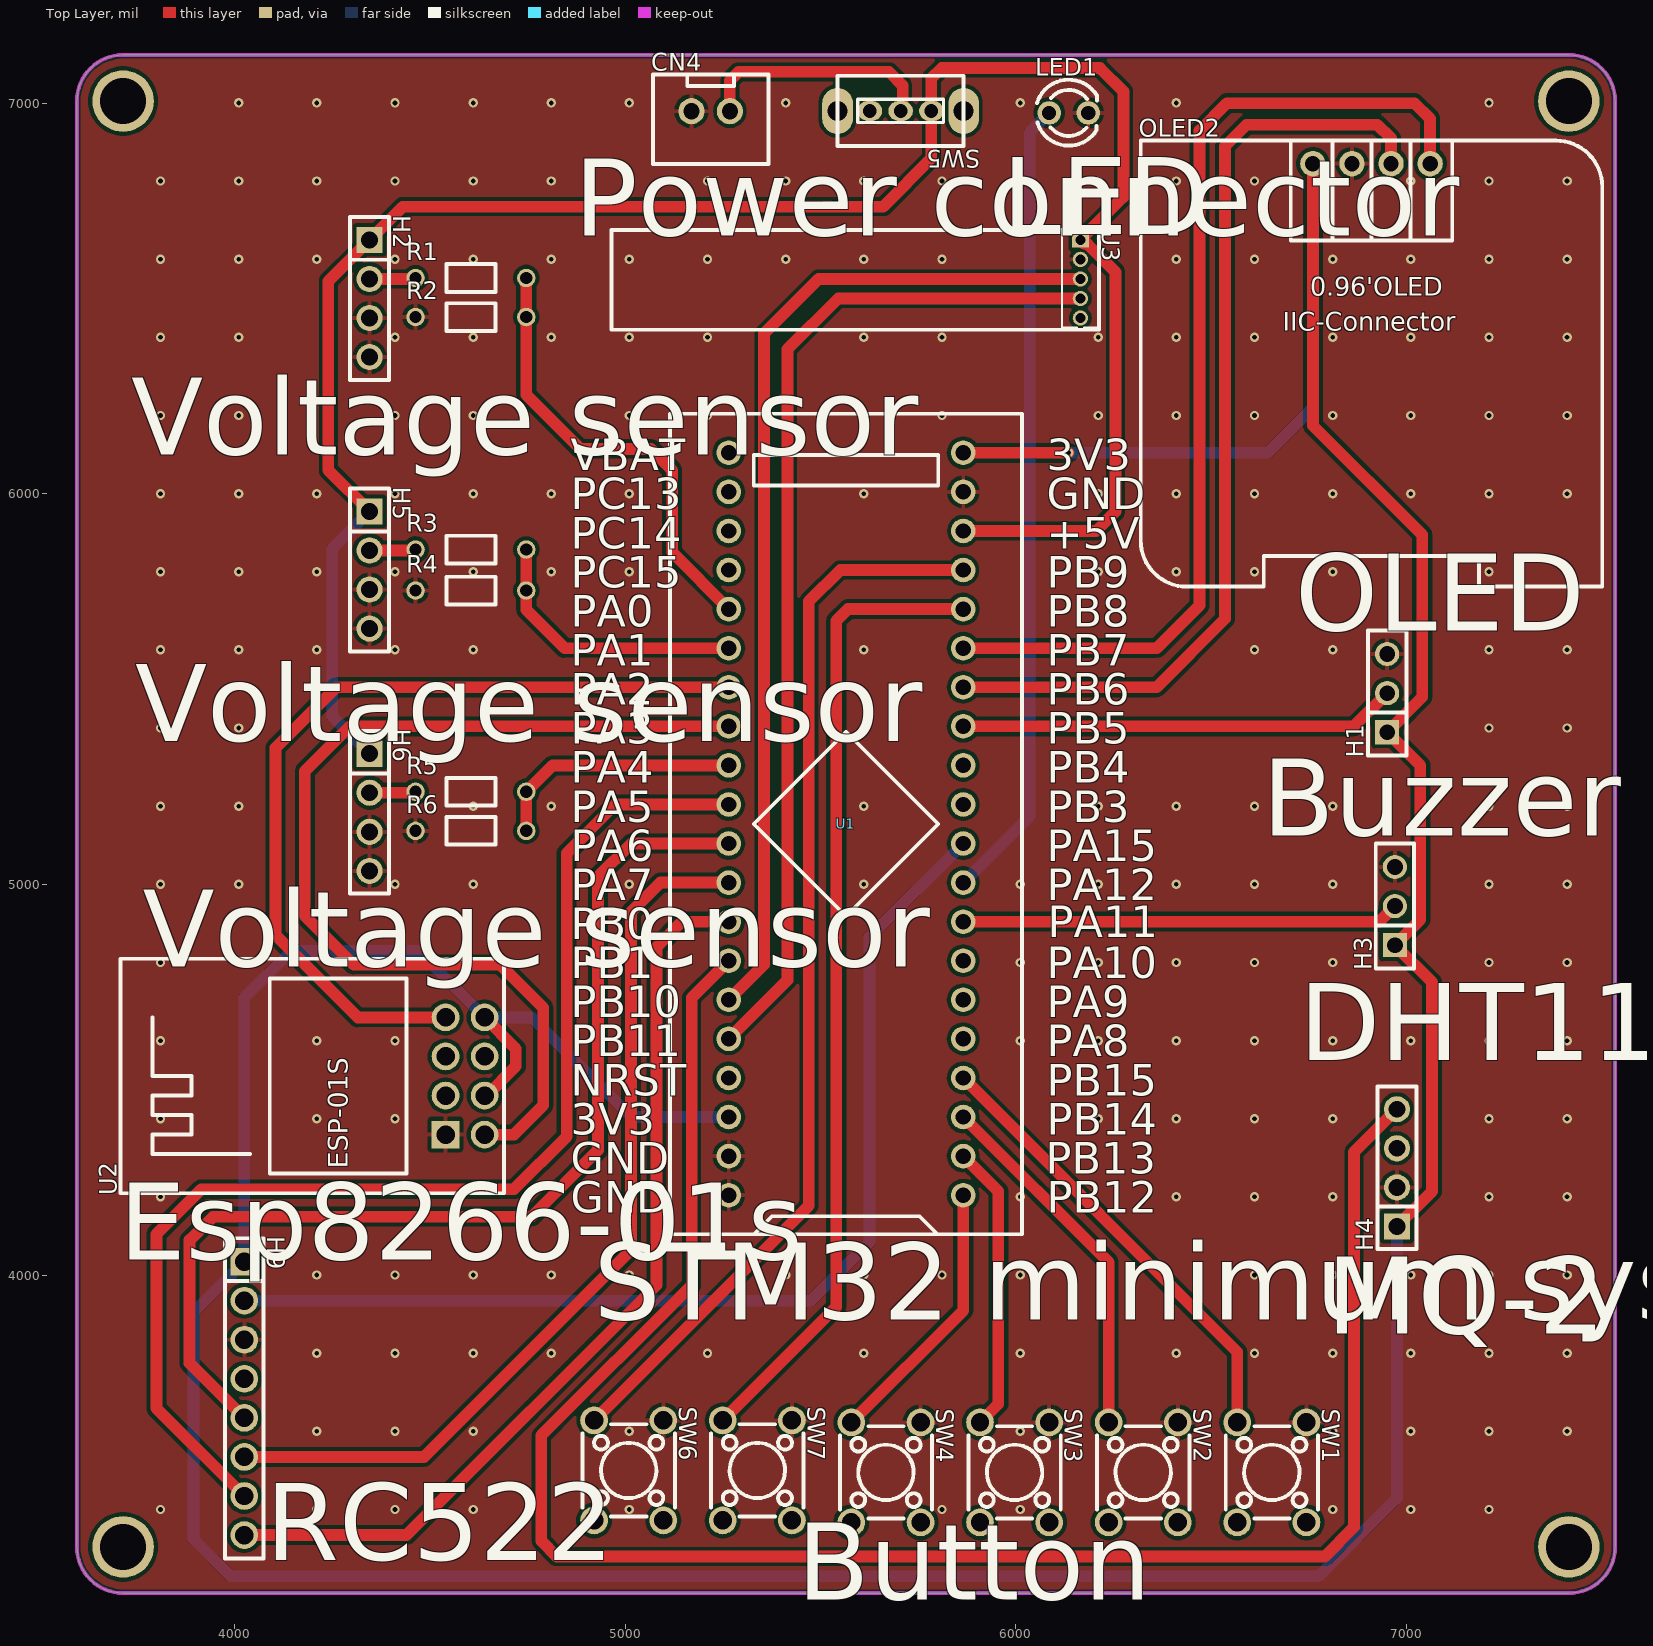
[diagram p0: Top Layer view]
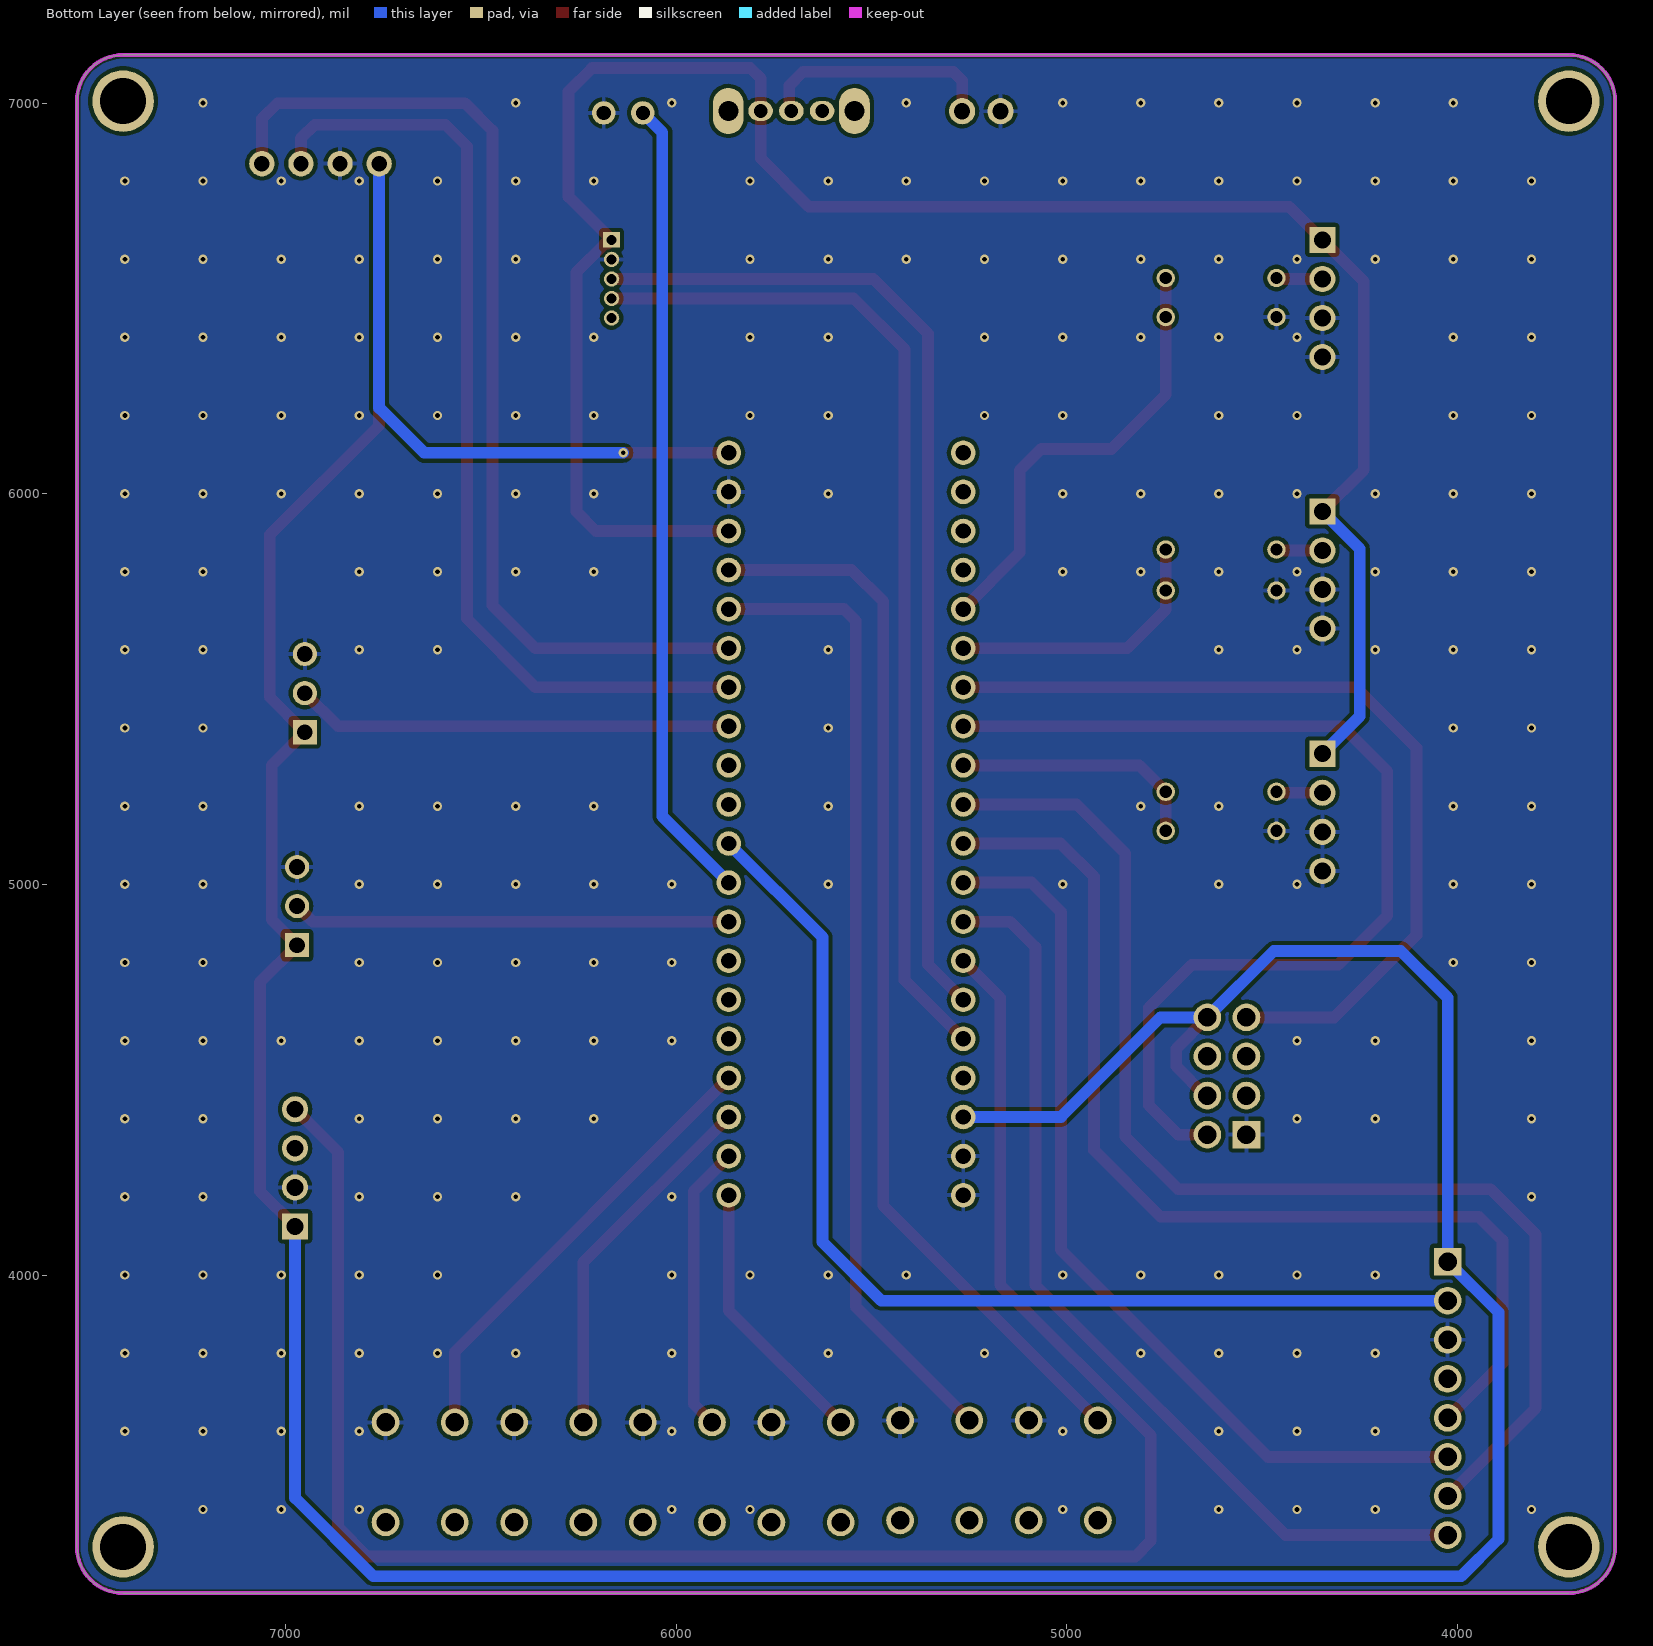
[diagram p1: Bottom Layer view, seen from below]
# Altium PCB MISC89009.pcbdoc
Units mil, origin at the board's own origin, x right, y up, seen from the top; angles counter-clockwise.
Board outline 3937.01 x 3937.01 mil, 2 copper layers (Top Layer, Bottom Layer), stack 62.206 mil thick; 26 components, 41 nets, 136 pads, 226 vias.

## Layer stack, top to bottom
Top Solder Mask Layer: solder mask 0.394, Dk 3.3
Top Layer: signal copper 1.379
Dielectric1: surface 59.449, FR4, Dk 4.5
Bottom Layer: signal copper 1.378
Bottom Solder Mask Layer: solder mask 0.394, Dk 3.3

## Board outline
3714.61,7123.5 ccw(c3714.61,7005.39) 3596.5,7005.39 3596.5,3304.61 ccw(c3714.61,3304.61) 3714.61,3186.5 7415.39,3186.5 ccw(c7415.39,3304.61) 7533.5,3304.61 7533.5,7005.39 ccw(c7415.39,7005.39) 7415.39,7123.5 3714.61,7123.5

## Design rules (kind name [scope] priority, off if disabled: settings)
BoardOutlineClearance copperThickness2oz_1 [All] p2 off: genericclearance=7.99 ignorepadtopadclearanceinfootprint=FALSE except(0: Arc-SplitContinuation Track-SplitContinuation SMDPad-SplitContinuation THPad-SplitContinuation Via-SplitContinuation Fill-SplitContinuation Region-SplitContinuation Poly-SplitContinuation Text-SplitContinuation Hole-SplitContinuation; 5.98: Arc-CutoutEdge Track-CutoutEdge SMDPad-CutoutEdge THPad-CutoutEdge Via-CutoutEdge Text-CutoutEdge; 6.9: Hole-OutlineEdge Hole-CutoutEdge; 10: Poly-OutlineEdge Poly-CutoutEdge; 11.81: Arc-OutlineEdge Track-OutlineEdge SMDPad-OutlineEdge THPad-OutlineEdge Via-OutlineEdge Fill-OutlineEdge Region-OutlineEdge Text-OutlineEdge Fill-CutoutEdge Region-CutoutEdge)
BoardOutlineClearance Plane_innerPlane_1 [All] p4 off: genericclearance=4.02 ignorepadtopadclearanceinfootprint=FALSE except(0: Arc-SplitContinuation Track-SplitContinuation SMDPad-SplitContinuation THPad-SplitContinuation Via-SplitContinuation Fill-SplitContinuation Region-SplitContinuation Poly-SplitContinuation Text-SplitContinuation Hole-SplitContinuation; 5.98: Arc-CutoutEdge Track-CutoutEdge SMDPad-CutoutEdge THPad-CutoutEdge Via-CutoutEdge Text-CutoutEdge; 6.9: Hole-OutlineEdge Hole-CutoutEdge; 10: Poly-OutlineEdge Poly-CutoutEdge; 11.81: Arc-OutlineEdge Track-OutlineEdge SMDPad-OutlineEdge THPad-OutlineEdge Via-OutlineEdge Fill-OutlineEdge Region-OutlineEdge Text-OutlineEdge Fill-CutoutEdge Region-CutoutEdge)
BoardOutlineClearance Copper_copperRegion_1 [All] p6 off: genericclearance=4.02 ignorepadtopadclearanceinfootprint=FALSE except(0: Arc-SplitContinuation Track-SplitContinuation SMDPad-SplitContinuation THPad-SplitContinuation Via-SplitContinuation Fill-SplitContinuation Region-SplitContinuation Poly-SplitContinuation Text-SplitContinuation Hole-SplitContinuation; 5.98: Arc-CutoutEdge Track-CutoutEdge SMDPad-CutoutEdge THPad-CutoutEdge Via-CutoutEdge Text-CutoutEdge; 6.9: Hole-OutlineEdge Hole-CutoutEdge; 10: Poly-OutlineEdge Poly-CutoutEdge; 11.81: Arc-OutlineEdge Track-OutlineEdge SMDPad-OutlineEdge THPad-OutlineEdge Via-OutlineEdge Fill-OutlineEdge Region-OutlineEdge Text-OutlineEdge Fill-CutoutEdge Region-CutoutEdge)
BoardOutlineClearance Copper_copperRegion_copperThickness1oz_1 [All] p8 off: genericclearance=4.02 ignorepadtopadclearanceinfootprint=FALSE except(0: Arc-SplitContinuation Track-SplitContinuation SMDPad-SplitContinuation THPad-SplitContinuation Via-SplitContinuation Fill-SplitContinuation Region-SplitContinuation Poly-SplitContinuation Text-SplitContinuation Hole-SplitContinuation; 5.98: Arc-CutoutEdge Track-CutoutEdge SMDPad-CutoutEdge THPad-CutoutEdge Via-CutoutEdge Text-CutoutEdge; 6.9: Hole-OutlineEdge Hole-CutoutEdge; 10: Poly-OutlineEdge Poly-CutoutEdge; 11.81: Arc-OutlineEdge Track-OutlineEdge SMDPad-OutlineEdge THPad-OutlineEdge Via-OutlineEdge Fill-OutlineEdge Region-OutlineEdge Text-OutlineEdge Fill-CutoutEdge Region-CutoutEdge)
BoardOutlineClearance Copper_copperRegion_Copper_copperRegion_1 [All] p10 off: genericclearance=4.02 ignorepadtopadclearanceinfootprint=FALSE except(0: Arc-SplitContinuation Track-SplitContinuation SMDPad-SplitContinuation THPad-SplitContinuation Via-SplitContinuation Fill-SplitContinuation Region-SplitContinuation Poly-SplitContinuation Text-SplitContinuation Hole-SplitContinuation; 5.98: Arc-CutoutEdge Track-CutoutEdge SMDPad-CutoutEdge THPad-CutoutEdge Via-CutoutEdge Text-CutoutEdge; 6.9: Hole-OutlineEdge Hole-CutoutEdge; 10: Poly-OutlineEdge Poly-CutoutEdge; 11.81: Arc-OutlineEdge Track-OutlineEdge SMDPad-OutlineEdge THPad-OutlineEdge Via-OutlineEdge Fill-OutlineEdge Region-OutlineEdge Text-OutlineEdge Fill-CutoutEdge Region-CutoutEdge)
BoardOutlineClearance copperThickness1oz_1 [All] p12: genericclearance=4.02 ignorepadtopadclearanceinfootprint=FALSE except(0: Arc-SplitContinuation Track-SplitContinuation SMDPad-SplitContinuation THPad-SplitContinuation Via-SplitContinuation Fill-SplitContinuation Region-SplitContinuation Poly-SplitContinuation Text-SplitContinuation Hole-SplitContinuation; 5.98: Arc-CutoutEdge Track-CutoutEdge SMDPad-CutoutEdge THPad-CutoutEdge Via-CutoutEdge Text-CutoutEdge; 6.9: Hole-OutlineEdge Hole-CutoutEdge; 10: Poly-OutlineEdge Poly-CutoutEdge; 11.81: Arc-OutlineEdge Track-OutlineEdge SMDPad-OutlineEdge THPad-OutlineEdge Via-OutlineEdge Fill-OutlineEdge Region-OutlineEdge Text-OutlineEdge Fill-CutoutEdge Region-CutoutEdge)
Clearance copperThickness2oz [All] p1 off: gap=7.99 ignorepadtopadclearanceinfootprint=FALSE except(5.98: SMDPad-Track SMDPad-SMDPad THPad-Track SMDPad-THPad THPad-THPad Track-Via SMDPad-Via THPad-Via Via-Via Fill-SMDPad Region-SMDPad Fill-THPad Region-THPad Fill-Via Region-Via Fill-Fill Fill-Region Region-Region Arc-Track Arc-SMDPad Arc-THPad Arc-Via Fill-Arc Region-Arc Arc-Arc Text-Track SMDPad-Text Text-THPad Text-Via Fill-Text Region-Text Arc-Text Text-Text; 6.9: Hole-Track Hole-SMDPad Hole-THPad Hole-Via Fill-Hole Region-Hole Hole-Arc Hole-Text; 10: Poly-Track Poly-SMDPad Poly-THPad Poly-Via Poly-Fill Poly-Region Poly-Poly Poly-Arc Poly-Text Poly-Hole; 11.81: Fill-Track Region-Track)
Clearance Plane_innerPlane [All] p3 off: gap=4.02 ignorepadtopadclearanceinfootprint=FALSE except(5.98: SMDPad-Track SMDPad-SMDPad THPad-Track SMDPad-THPad THPad-THPad Track-Via SMDPad-Via THPad-Via Via-Via Fill-SMDPad Region-SMDPad Fill-THPad Region-THPad Fill-Via Region-Via Fill-Fill Fill-Region Region-Region Arc-Track Arc-SMDPad Arc-THPad Arc-Via Fill-Arc Region-Arc Arc-Arc Text-Track SMDPad-Text Text-THPad Text-Via Fill-Text Region-Text Arc-Text Text-Text; 6.9: Hole-Track Hole-SMDPad Hole-THPad Hole-Via Fill-Hole Region-Hole Hole-Arc Hole-Text; 10: Poly-Track Poly-SMDPad Poly-THPad Poly-Via Poly-Fill Poly-Region Poly-Poly Poly-Arc Poly-Text Poly-Hole; 11.81: Fill-Track Region-Track)
Clearance Copper_copperRegion [All] p5 off: gap=4.02 ignorepadtopadclearanceinfootprint=FALSE except(5.98: SMDPad-Track SMDPad-SMDPad THPad-Track SMDPad-THPad THPad-THPad Track-Via SMDPad-Via THPad-Via Via-Via Fill-SMDPad Region-SMDPad Fill-THPad Region-THPad Fill-Via Region-Via Fill-Fill Fill-Region Region-Region Arc-Track Arc-SMDPad Arc-THPad Arc-Via Fill-Arc Region-Arc Arc-Arc Text-Track SMDPad-Text Text-THPad Text-Via Fill-Text Region-Text Arc-Text Text-Text; 6.9: Hole-Track Hole-SMDPad Hole-THPad Hole-Via Fill-Hole Region-Hole Hole-Arc Hole-Text; 10: Poly-Track Poly-SMDPad Poly-THPad Poly-Via Poly-Fill Poly-Region Poly-Poly Poly-Arc Poly-Text Poly-Hole; 11.81: Fill-Track Region-Track)
Clearance Copper_copperRegion_copperThickness1oz [All] p7 off: gap=4.02 ignorepadtopadclearanceinfootprint=FALSE except(5.98: SMDPad-Track SMDPad-SMDPad THPad-Track SMDPad-THPad THPad-THPad Track-Via SMDPad-Via THPad-Via Via-Via Fill-SMDPad Region-SMDPad Fill-THPad Region-THPad Fill-Via Region-Via Fill-Fill Fill-Region Region-Region Arc-Track Arc-SMDPad Arc-THPad Arc-Via Fill-Arc Region-Arc Arc-Arc Text-Track SMDPad-Text Text-THPad Text-Via Fill-Text Region-Text Arc-Text Text-Text; 6.9: Hole-Track Hole-SMDPad Hole-THPad Hole-Via Fill-Hole Region-Hole Hole-Arc Hole-Text; 10: Poly-Track Poly-SMDPad Poly-THPad Poly-Via Poly-Fill Poly-Region Poly-Poly Poly-Arc Poly-Text Poly-Hole; 11.81: Fill-Track Region-Track)
Clearance Copper_copperRegion_Copper_copperRegion [All] p9 off: gap=4.02 ignorepadtopadclearanceinfootprint=FALSE except(5.98: SMDPad-Track SMDPad-SMDPad THPad-Track SMDPad-THPad THPad-THPad Track-Via SMDPad-Via THPad-Via Via-Via Fill-SMDPad Region-SMDPad Fill-THPad Region-THPad Fill-Via Region-Via Fill-Fill Fill-Region Region-Region Arc-Track Arc-SMDPad Arc-THPad Arc-Via Fill-Arc Region-Arc Arc-Arc Text-Track SMDPad-Text Text-THPad Text-Via Fill-Text Region-Text Arc-Text Text-Text; 6.9: Hole-Track Hole-SMDPad Hole-THPad Hole-Via Fill-Hole Region-Hole Hole-Arc Hole-Text; 10: Poly-Track Poly-SMDPad Poly-THPad Poly-Via Poly-Fill Poly-Region Poly-Poly Poly-Arc Poly-Text Poly-Hole; 11.81: Fill-Track Region-Track)
Clearance copperThickness1oz [All] p11: gap=4.02 ignorepadtopadclearanceinfootprint=FALSE except(5.98: SMDPad-Track SMDPad-SMDPad THPad-Track SMDPad-THPad THPad-THPad Track-Via SMDPad-Via THPad-Via Via-Via Fill-SMDPad Region-SMDPad Fill-THPad Region-THPad Fill-Via Region-Via Fill-Fill Fill-Region Region-Region Arc-Track Arc-SMDPad Arc-THPad Arc-Via Fill-Arc Region-Arc Arc-Arc Text-Track SMDPad-Text Text-THPad Text-Via Fill-Text Region-Text Arc-Text Text-Text; 6.9: Hole-Track Hole-SMDPad Hole-THPad Hole-Via Fill-Hole Region-Hole Hole-Arc Hole-Text; 10: Poly-Track Poly-SMDPad Poly-THPad Poly-Via Poly-Fill Poly-Region Poly-Poly Poly-Arc Poly-Text Poly-Hole; 11.81: Fill-Track Region-Track)
DiffPairsRouting differentialPair [All] p1: maxlimit=6 minlimit=6 mostfreqgap=6 toplayer_minwidth=5 toplayer_prefwidth=10 toplayer_maxwidth=100 toplayer_mingap=6 toplayer_prefgap=6 toplayer_maxgap=6 bottomlayer_minwidth=5 bottomlayer_prefwidth=10 bottomlayer_maxwidth=100 bottomlayer_mingap=6 bottomlayer_prefgap=6 bottomlayer_maxgap=6 maxuncoupledlength=10
HoleToHoleClearance otherClearance [All] p1: gap=11.81 allowstackedmicrovias=TRUE
Length netLength [All] p1: minlimit=0 maxlimit=0
PasteMaskExpansion pasteMaskExpansion [All] p1: expansion=0
PlaneConnect innerPlane [All] p1: planeconnectstyle=Relief reliefexpansion=20 reliefentries=4 reliefconductorwidth=10 reliefairgap=10
PolygonConnect copperRegion_copperThickness1oz [All] p1 off: connectstyle=Relief reliefconductorwidth=10 reliefentries=4 polygonreliefangle="90 Angle" airgapwidth=10 via.connectstyle=Relief via.reliefconductorwidth=10 via.reliefentries=4 via.polygonreliefangle="90 Angle" via.airgapwidth=10
PolygonConnect copperRegion_Copper_copperRegion [All] p2 off: connectstyle=Relief reliefconductorwidth=10 reliefentries=4 polygonreliefangle="90 Angle" airgapwidth=10 via.connectstyle=Relief via.reliefconductorwidth=10 via.reliefentries=4 via.polygonreliefangle="90 Angle" via.airgapwidth=10
PolygonConnect copperRegion [All] p3: connectstyle=Relief reliefconductorwidth=10 reliefentries=4 polygonreliefangle="90 Angle" airgapwidth=10 via.connectstyle=Relief via.reliefconductorwidth=10 via.reliefentries=4 via.polygonreliefangle="90 Angle" via.airgapwidth=10
RoutingVias viaSize [All] p1: holewidth=12.01 width=24.02 viastyle="Through Hole" minholewidth=11.81 minwidth=19.68 maxholewidth=248.03 maxwidth=393.7
SolderMaskExpansion solderMaskExpansion [IsVia] p1: expansion=-1000 istentingtop=TRUE
SolderMaskExpansion solderMaskExpansion [All] p2: expansion=2 istentingtop=FALSE
Width copperThickness2oz_2 [All] p1 off: maxlimit=100 minlimit=8 preferedwidth=10
Width copperThickness1oz_2 [All] p2: maxlimit=100 minlimit=5 preferedwidth=10

## Components (designator, comment, footprint, x,y, rotation, side; value= is the part's Value field where it differs from the comment)
CN4 "XH2.54*2P_THT" CONN-TH_2P-P2.50-XH2.54-2P 5218.59,6979.34 r0 top
H1 "" HDR-TH_3P-P2.54-V-F 6950,5490 r90 top
H2 "" HDR-TH_4P-P2.54-V-F 4345.79,6499.99 r270 top
H3 "" HDR-TH_3P-P2.54-V-F 6970,4945 r90 top
H4 "" HDR-TH_4P-P2.54-V-F 6975,4275 r90 top
H5 "" HDR-TH_4P-P2.54-V-F 4345.79,5804.99 r270 top
H6 "" HDR-TH_4P-P2.54-V-F 4345.79,5184.99 r270 top
H9 "" HDR-TH_8P-P2.54-V-F-1 4025,3685 r270 top
LED1 "" LED_TH-3mm 6135,6975 r0 top
OLED2 "" 0.96OLED_4P 6910,6845 r0 top
R1 "10kΩ" Res_1/8W 4605,6550 r0 top
R2 "6.8kΩ" Res_1/8W 4605,6450 r0 top
R3 "10kΩ" Res_1/8W 4605,5855 r0 top
R4 "6.8kΩ" Res_1/8W 4605,5750 r0 top
R5 "10kΩ" Res_1/8W 4605,5235 r0 top
R6 "6.8kΩ" Res_1/8W 4605,5135 r0 top
SW1 "" SW-TH_4P-L6.0-W6.0-P4.50-LS6.5 6654.94,3495.48 r270 top
SW2 "" SW-TH_4P-L6.0-W6.0-P4.50-LS6.5 6325.72,3495.48 r270 top
SW3 "" SW-TH_4P-L6.0-W6.0-P4.50-LS6.5 5996.5,3495.48 r270 top
SW4 "" SW-TH_4P-L6.0-W6.0-P4.50-LS6.5 5667.28,3495.48 r270 top
SW5 "" 拨动开关 5710,6980 r180 top
SW6 "" SW-TH_4P-L6.0-W6.0-P4.50-LS6.5 5008.84,3500.48 r270 top
SW7 "" SW-TH_4P-L6.0-W6.0-P4.50-LS6.5 5338.06,3500.48 r270 top
U1 "STM32F103C8T6-Card" CONN-TH_L53.3-W22.9_STM32F103C8T6-CARD 5565,5155 r90 top
U2 "ESP-01S" WIFIM-TH_ESP-01S 4590,4510 r90 top
U3 "FPH12728-S05S1014190140B" HDR-TH_5P-P1.27-V-M-1 6165,6550 r270 top

## Footprints (in the part's own frame and the unit in brackets; to place one, negate y for a bottom-side part, rotate by r counter-clockwise, add the part's x,y. Pads: shape width x height; smd on the part's side, far side on the other; paste and mask are expansions set on the pad)
0.96OLED_4P [mm]
  round 1.65 hole 1 copper offset 0,0: 1(-3.81,-0.001) 2(-1.27,0.002) 3(1.27,0.002) 4(3.81,0.002)
  silkscreen extent -15,-27.5 15,1.5
CONN-TH_2P-P2.50-XH2.54-2P [mm]
  round 1.7 hole 1.05 paste+0 mask+0.05: 1(1.25,0) 2(-1.25,0)
  silkscreen extent -3.75,-3.42 3.75,2.37
CONN-TH_L53.3-W22.9_STM32F103C8T6-CARD [mm]
  round 1.6 hole 1: 1(-24.13,-7.62) 2(-21.59,-7.62) 3(-19.05,-7.62) 4(-16.51,-7.62) 5(-13.97,-7.62) 6(-11.43,-7.62) 7(-8.89,-7.62) 8(-6.35,-7.62) 9(-3.81,-7.62) 10(-1.27,-7.62) 11(1.27,-7.62) 12(3.81,-7.62) 13(6.35,-7.62) 14(8.89,-7.62) 15(11.43,-7.62) 16(13.97,-7.62) 17(16.51,-7.62) 18(19.05,-7.62) 19(21.59,-7.62) 20(24.13,-7.62) 21(24.13,7.62) 22(21.59,7.62) 23(19.05,7.62) 24(16.51,7.62) 25(13.97,7.62) 26(11.43,7.62) 27(8.89,7.62) 28(6.35,7.62) 29(3.81,7.62) 30(1.27,7.62) 31(-1.27,7.62) 32(-3.81,7.62) 33(-6.35,7.62) 34(-8.89,7.62) 35(-11.43,7.62) 36(-13.97,7.62) 37(-16.51,7.62) 38(-19.05,7.62) 39(-21.59,7.62) 40(-24.13,7.62)
  silkscreen extent -26.67,-11.43 26.67,11.43
HDR-TH_3P-P2.54-V-F [mil]
  rect 62x62 hole 40.16: 1(-100,0)
  round 62 hole 40.16: 2(0,0) 3(100,0)
  silkscreen extent -160,-49 160,49
HDR-TH_4P-P2.54-V-F [mm]
  rect 1.7x1.7 hole 1.1: 1(-3.81,0)
  round 1.7 hole 1.1: 2(-1.27,0) 3(1.27,0) 4(3.81,0)
  silkscreen extent -5.29,-1.27 5.29,1.27
HDR-TH_5P-P1.27-V-M-1 [mm]
  rect 1x1.1 hole 0.65: 1(-2.54,0)
  round 1 hole 0.65: 2(-1.27,0) 3(0,0) 4(1.27,0) 5(2.54,0)
  silkscreen extent -3.18,-1.2 3.18,1.2
HDR-TH_8P-P2.54-V-F-1 [mm]
  rect 1.8x1.8 hole 1.2: 1(-8.89,0)
  round 1.8 hole 1.2: 2(-6.35,0) 3(-3.81,0) 4(-1.27,0) 5(1.27,0) 6(3.81,0) 7(6.35,0) 8(8.89,0)
  silkscreen extent -10.41,-1.25 10.41,1.25
LED_TH-3mm [mil]
  round 60 hole 36 paste+0 mask+2: 1(-50,0) 2(50,0)
  silkscreen extent -81,-84 72,85
Res_1/8W [mil]
  round 47.2 hole 31.5 paste+0 mask+2: 1(-141.7,2.48) 2(141.7,2.48)
  silkscreen extent -63,-33 63,38
SW-TH_4P-L6.0-W6.0-P4.50-LS6.5 [mm]
  round 1.8 hole 1.2: 1(-3.25,2.25) 2(3.25,2.25) 3(-3.25,-2.25) 4(3.25,-2.25)
  silkscreen extent -3,-3 3,3
WIFIM-TH_ESP-01S [mm]
  rect 1.8x1.8 hole 1.2: 1(-3.81,1.27)
  round 1.8 hole 1.2: 2(-1.27,1.27) 3(1.27,1.27) 4(3.81,1.27) 5(3.81,-1.27) 6(1.27,-1.27) 7(-1.27,-1.27) 8(-3.81,-1.27)
  silkscreen extent -7.62,-2.54 7.62,22.4
拨动开关 [mil]
  oval 63x51.2 hole 35.4 paste+0 mask+2: 1(-73.4,0) 2(5,0) 3(84,0)
  oval 78.7x118.1 hole 51.2 paste+0 mask+2: 4(166.7,0) 5(-156.1,0)
  silkscreen extent -156,-90 167,90

## Free pads (board coordinates)
  round 157.48 hole 118.11: 1(3714.61,7005.39) 1(3714.61,3304.61) 1(7415.39,7005.39) 1(7415.39,3304.61)

## Via types
v1: diameter 24.02, hole 12, Top Layer to Bottom Layer, 226 vias

## Nets (pads, with @x,y where several pads share a name; then routed paths per layer and width w, separated by ;. In a path a pad name is that pad's centre, name@x,y a point inside that pad or via, vN(x,y) a via of type N, cw(c..) or ccw(c..) an arc to the next point about the centre after c; other vN are vias at no path point)
$1N17118: CN4.1 SW5.2 | length 611.4
  Top Layer w30: CN4.1 5267.8,7057.8 5290,7080 5675,7080 5710,7045 5710,6985 SW5.2
$1N17383: H2.2 R1.1 | length 118.5
  Top Layer w30: H2.2 4460.81,6549.99 R1.1
$1N17388: H5.2 R3.1 | length 118.5
  Top Layer w30: H5.2 4460.81,5854.99 R3.1
$1N17392: H6.2 R5.1 | length 118.5
  Top Layer w30: H6.2 4460.81,5234.99 R5.1
+5V: H2.1 H5.1 H6.1 SW5.1 U1.18 U3.1 | length 5311.4
  Top Layer w30: H5.1 4240,6060.78 4240,6544.2 H2.1 4430.8,6735 5660,6735 5783.4,6858.4 SW5.1 5783.4,7063.4 5810,7090 6215,7090 6275,7030 6275,6760 U3.1 6174.33,6640.67 6181.85,6640.67 6255,6567.52 6255,5955 6205,5905 U1.18
  Bottom Layer w30: H6.1 4250,5430.78 4250,5859.2 H5.1
GND: CN4.2 H1.3 H2.3 H2.4 H3.3 H4.2 H5.3 H5.4 H6.3 H6.4 H9.3 LED1.2 OLED2.2 R2.1 R4.1 R6.1 SW1.1 SW2.1 SW3.1 SW4.1 SW6.1 SW7.1 U1.19 U1.39 U1.40 U2.1 U3.2
  other v1: 3810.6,3400.6 4210.6,3400.6 4410.6,3400.6 4610.6,3400.6 5010.6,3400.6 5810.6,3400.6 6010.6,3400.6 6810.6,3400.6 7010.6,3400.6 7210.6,3400.6 4210.6,3600.6 4410.6,3600.6 4610.6,3600.6 5010.6,3600.6 6010.6,3600.6 6810.6,3600.6 7010.6,3600.6 7210.6,3600.6 7410.6,3600.6 4210.6,3800.6 4410.6,3800.6 4610.6,3800.6 4810.6,3800.6 5210.6,3800.6 5610.6,3800.6 6010.6,3800.6 6410.6,3800.6 6610.6,3800.6 6810.6,3800.6 7010.6,3800.6 7210.6,3800.6 7410.6,3800.6 4210.6,4000.6 4410.6,4000.6 4610.6,4000.6 4810.6,4000.6 5010.6,4000.6 5410.6,4000.6 5610.6,4000.6 5810.6,4000.6 6010.6,4000.6 6610.6,4000.6 6810.6,4000.6 7010.6,4000.6 7210.6,4000.6 7410.6,4000.6 3810.6,4200.6 6010.6,4200.6 6410.6,4200.6 6610.6,4200.6 6810.6,4200.6 7210.6,4200.6 7410.6,4200.6 3810.6,4400.6 4210.6,4400.6 4410.6,4400.6 6210.6,4400.6 6410.6,4400.6 6610.6,4400.6 6810.6,4400.6 7210.6,4400.6 7410.6,4400.6 3810.6,4600.6 4210.6,4600.6 4410.6,4600.6 6010.6,4600.6 6210.6,4600.6 6410.6,4600.6 6610.6,4600.6 6810.6,4600.6 7010.6,4600.6 7210.6,4600.6 7410.6,4600.6 3810.6,4800.6 4010.6,4800.6 6010.6,4800.6 6210.6,4800.6 6410.6,4800.6 6610.6,4800.6 6810.6,4800.6 7210.6,4800.6 7410.6,4800.6 3810.6,5000.6 4010.6,5000.6 4410.6,5000.6 4610.6,5000.6 5010.6,5000.6 5610.6,5000.6 6010.6,5000.6 6210.6,5000.6 6410.6,5000.6 6610.6,5000.6 6810.6,5000.6 7210.6,5000.6 7410.6,5000.6 3810.6,5200.6 4010.6,5200.6 4610.6,5200.6 4810.6,5200.6 5610.6,5200.6 6210.6,5200.6 6410.6,5200.6 6610.6,5200.6 6810.6,5200.6 7210.6,5200.6 7410.6,5200.6 3810.6,5400.6 4010.6,5400.6 5610.6,5400.6 7210.6,5400.6 7410.6,5400.6 3810.6,5600.6 4010.6,5600.6 4210.6,5600.6 4410.6,5600.6 4610.6,5600.6 5610.6,5600.6 6610.6,5600.6 6810.6,5600.6 7210.6,5600.6 7410.6,5600.6 3810.6,5800.6 4010.6,5800.6 4210.6,5800.6 4410.6,5800.6 4610.6,5800.6 4810.6,5800.6 5010.6,5800.6 6210.6,5800.6 6410.6,5800.6 6610.6,5800.6 6810.6,5800.6 7210.6,5800.6 7410.6,5800.6 3810.6,6000.6 4010.6,6000.6 4210.6,6000.6 4410.6,6000.6 4610.6,6000.6 4810.6,6000.6 5010.6,6000.6 5610.6,6000.6 6210.6,6000.6 6410.6,6000.6 6610.6,6000.6 6810.6,6000.6 7010.6,6000.6 7210.6,6000.6 7410.6,6000.6 3810.6,6200.6 4010.6,6200.6 4410.6,6200.6 4610.6,6200.6 5010.6,6200.6 5210.6,6200.6 5610.6,6200.6 5810.6,6200.6 6210.6,6200.6 6410.6,6200.6 6610.6,6200.6 6810.6,6200.6 7010.6,6200.6 7210.6,6200.6 7410.6,6200.6 3810.6,6400.6 4010.6,6400.6 4410.6,6400.6 4610.6,6400.6 4810.6,6400.6 5010.6,6400.6 5210.6,6400.6 5610.6,6400.6 5810.6,6400.6 6210.6,6400.6 6410.6,6400.6 6610.6,6400.6 6810.6,6400.6 7010.6,6400.6 7210.6,6400.6 7410.6,6400.6 3810.6,6600.6 4010.6,6600.6 4210.6,6600.6 4410.6,6600.6 4610.6,6600.6 4810.6,6600.6 5010.6,6600.6 5210.6,6600.6 5410.6,6600.6 5610.6,6600.6 5810.6,6600.6 6410.6,6600.6 6610.6,6600.6 6810.6,6600.6 7010.6,6600.6 7210.6,6600.6 7410.6,6600.6 3810.6,6800.6 4010.6,6800.6 4210.6,6800.6 4410.6,6800.6 4610.6,6800.6 4810.6,6800.6 5010.6,6800.6 5210.6,6800.6 5410.6,6800.6 5610.6,6800.6 5810.6,6800.6 6210.6,6800.6 6410.6,6800.6 6610.6,6800.6 6810.6,6800.6 7010.6,6800.6 7210.6,6800.6 7410.6,6800.6 4010.6,7000.6 4210.6,7000.6 4410.6,7000.6 4610.6,7000.6 4810.6,7000.6 5010.6,7000.6 5410.6,7000.6 6010.6,7000.6 6410.6,7000.6 7210.6,7000.6
NRST: U1.37
PA0: R1.2 R2.2 U1.25 | length 1167.6
  Top Layer w30: R1.2 R2.2 4746.7,6253.3 4885,6115 5065,6115 5120,6060 5120,5850 U1.25
PA1: R3.2 R4.2 U1.26 | length 713.2
  Top Layer w30: R3.2 R4.2 4746.7,5703.3 4845,5605 U1.26
PA2: U1.27 U2.4 | length 2226.2
  Top Layer w30: U2.4 4315,4660 4105,4870 4105,5350 4260,5505 U1.27
PA3: U1.28 U2.8 | length 2641
  Top Layer w30: U2.8 4715,4360 4790,4435 4790,4685 4680,4795 4305,4795 4180,4920 4180,5290 4295,5405 U1.28
PA4: R5.2 R6.2 U1.29 | length 646.3
  Top Layer w30: R6.2 R5.2 4814.23,5305 U1.29
PA5: H9.7 U1.30 | length 3108.5
  Top Layer w30: H9.7 3800,3660 3800,4105 3915,4220 4715,4220 4850,4355 4850,5080 4975,5205 U1.30
PA6: H9.5 U1.31 | length 2723.5
  Top Layer w30: H9.5 3885,3775 3885,4090 3945,4150 4760,4150 4930,4320 4930,5020 5015,5105 U1.31
PA7: H9.6 U1.32 | length 2355.6
  Top Layer w30: H9.6 4485,3535 5015,4065 5015,4930 5090,5005 U1.32
PA8: U1.5
PA9: U1.6
PA10: U1.7
PA11: H3.2 U1.8 | length 1121.6
  Top Layer w30: U1.8 6930,4905 H3.2
PA12: LED1.1 U1.9 | length 2061.1
  Bottom Layer w30: U1.9 6035,5175 6035,6925 LED1.1
PA15: H9.2 U1.10 | length 2781.5
  Bottom Layer w30: H9.2 5475,3935 5625,4085 5625,4865 U1.10
PB0: H9.8 U1.33 | length 2397
  Top Layer w30: H9.8 4440,3335 5080,3975 5080,4840 5145,4905 U1.33
PB1: H4.4 U1.34 | length 4927
  Top Layer w30: U1.34 5170,4710 5170,3975 4785,3590 4785,3320 4825,3280 6790,3280 6865,3355 6865,4315 H4.4
PB3: U1.11
PB4: U1.12
PB5: H1.2 U1.13 | length 1120.2
  Top Layer w30: U1.13 6865,5405 H1.2
PB6: OLED2.3 U1.14 | length 2479.7
  Top Layer w30: U1.14 6360,5505 6535,5680 6535,6890 6590,6945 6925,6945 6960,6910 OLED2.3@6960,6845.05
PB7: OLED2.4 U1.15 | length 2616.1
  Top Layer w30: U1.15 6360,5605 6470,5715 6470,6930 6540,7000 7020,7000 7060,6960 OLED2.4@7060,6845.05
PB8: SW7.3 U1.16 | length 2504.3
  Top Layer w30: SW7.3 5540,3918.96 5540,5675 5570,5705 U1.16
PB9: SW6.3 U1.17 | length 2752.4
  Top Layer w30: SW6.3 5470,4178.18 5470,5725 5550,5805 U1.17
PB10: U1.35 U3.3 | length 2610.3
  Top Layer w30: U1.35 5355,4795 5355,6410 5495,6550 U3.3
PB11: U1.36 U3.4 | length 2631
  Top Layer w30: U1.36 5415,4755 5415,6370 5545,6500 U3.4
PB12: SW4.3 U1.1 | length 700.2
  Top Layer w30: SW4.3 5865,3909.73 U1.1
PB13: SW3.3 U1.2 | length 738.3
  Top Layer w30: U1.2 5955,4215 5955,3670.51 SW3.3
PB14: SW2.3 U1.3 | length 935.7
  Top Layer w30: U1.3 6237.14,4032.86 SW2.3
PB15: SW1.3 U1.4 | length 1172.1
  Top Layer w30: U1.4 6566.36,3803.64 SW1.3
PC13: U1.22
PC14: U1.23
PC15: U1.24
VBAT: U1.21
VCC: H1.1 H3.1 H4.1 H9.1 OLED2.1 U1.20 U1.38 U2.5 U2.7 | length 11650.5
  Top Layer w30: U2.7 4645,4460 4720,4535 4720,4580 U2.5 ; U1.20 v1(6135,6105) ; OLED2.1 6760,6175 7040,5895 7040,5480 H1.1 7035,5305 7035,4910 H3.1 7065,4750 7065,4215 H4.1
  Bottom Layer w30: U1.38 5015,4405 4760,4660 U2.5 4470,4830 4145,4830 4025,4710 H9.1 3895,3905 3895,3325 3990,3230 6775,3230 6975,3430 H4.1 ; v1(6135,6105) 6645,6105 6760,6220 OLED2.1
pads on no net: H4.3 H9.4 SW1.2 SW1.4 SW2.2 SW2.4 SW3.2 SW3.4 SW4.2 SW4.4 SW5.3 SW5.4 SW5.5 SW6.2 SW6.4 SW7.2 SW7.4 U2.2 U2.3 U2.6 U3.5

## Polygon pours and split planes (outlines as drawn)
GND on Bottom Layer (solid, remove dead copper, pour order 2): 3525,7245 3525,3080 7700,3080 7700,7245
GND on Top Layer (solid, remove dead copper, pour order 2): 3000,7415 3000,3000 7930,3000 7930,7415

## Keep-outs
Board Outline Layer:
  the board outline again, w10

## Silkscreen, mask and mechanical layers (free items; w line width, h text height)
Top Silkscreen Layer:
  lines w10: 4965,6420 4965,6675 6212.24,6675 6212.24,6420 4965,6420
  text "LED" at 5965,6665 h196.85
  text "Power connector" at 4870,6660 h196.85
  text "Voltage sensor" at 3735,6100 h196.85
  text "VBAT" at 4860.95,6060 h80
  text "3V3" at 6079.16,6060 h80
  text "PC13" at 4860.95,5960 h80
  text "GND" at 6079.16,5960 h80
  text "PC14" at 4860.95,5860 h80
  text "+5V" at 6079.16,5860 h80
  text "PC15" at 4860.95,5760 h80
  text "PB9" at 6079.16,5760 h80
  text "PA0" at 4860.95,5660 h80
  text "PB8" at 6079.16,5660 h80
  text "OLED" at 6715,5650 h196.85
  text "PA1" at 4860.95,5560 h80
  text "PB7" at 6079.16,5560 h80
  text "PA2" at 4860.95,5460 h80
  text "PB6" at 6079.16,5460 h80
  text "Voltage sensor" at 3745.24,5366.57 h196.85
  text "PA3" at 4860.95,5360 h80
  text "PB5" at 6079.16,5360 h80
  text "PA4" at 4860.95,5260 h80
  text "PB4" at 6079.16,5260 h80
  text "PA5" at 4860.95,5160 h80
  text "PB3" at 6079.16,5160 h80
  text "Buzzer" at 6630,5125 h196.85
  text "PA6" at 4860.95,5060 h80
  text "PA15" at 6079.16,5060 h80
  text "PA7" at 4860.95,4960 h80
  text "PA12" at 6079.16,4960 h80
  text "PA11" at 6080.95,4865 h80
  text "PB0" at 4860.95,4860 h80
  text "Voltage sensor" at 3765,4790 h196.85
  text "PB1" at 4860.95,4760 h80
  text "PA10" at 6079.16,4760 h80
  text "PB10" at 4860.95,4660 h80
  text "PA9" at 6079.16,4660 h80
  text "PB11" at 4860.95,4560 h80
  text "PA8" at 6079.16,4560 h80
  text "DHT11" at 6725,4550 h196.85
  text "NRST" at 4860.95,4460 h80
  text "PB15" at 6079.16,4460 h80
  text "3V3" at 4860.95,4360 h80
  text "PB14" at 6079.16,4360 h80
  text "GND" at 4860.95,4260 h80
  text "PB13" at 6075.95,4260 h80
  text "GND" at 4860.95,4160 h80
  text "PB12" at 6079.16,4160 h80
  text "Esp8266-01s" at 3705,4040 h196.85
  text "STM32 minimum system" at 4919.45,3886.57 h196.85
  text "MQ-2" at 6795,3850 h196.85
  text "RC522" at 4080,3270 h196.85
  text "Button" at 5440,3170 h196.85